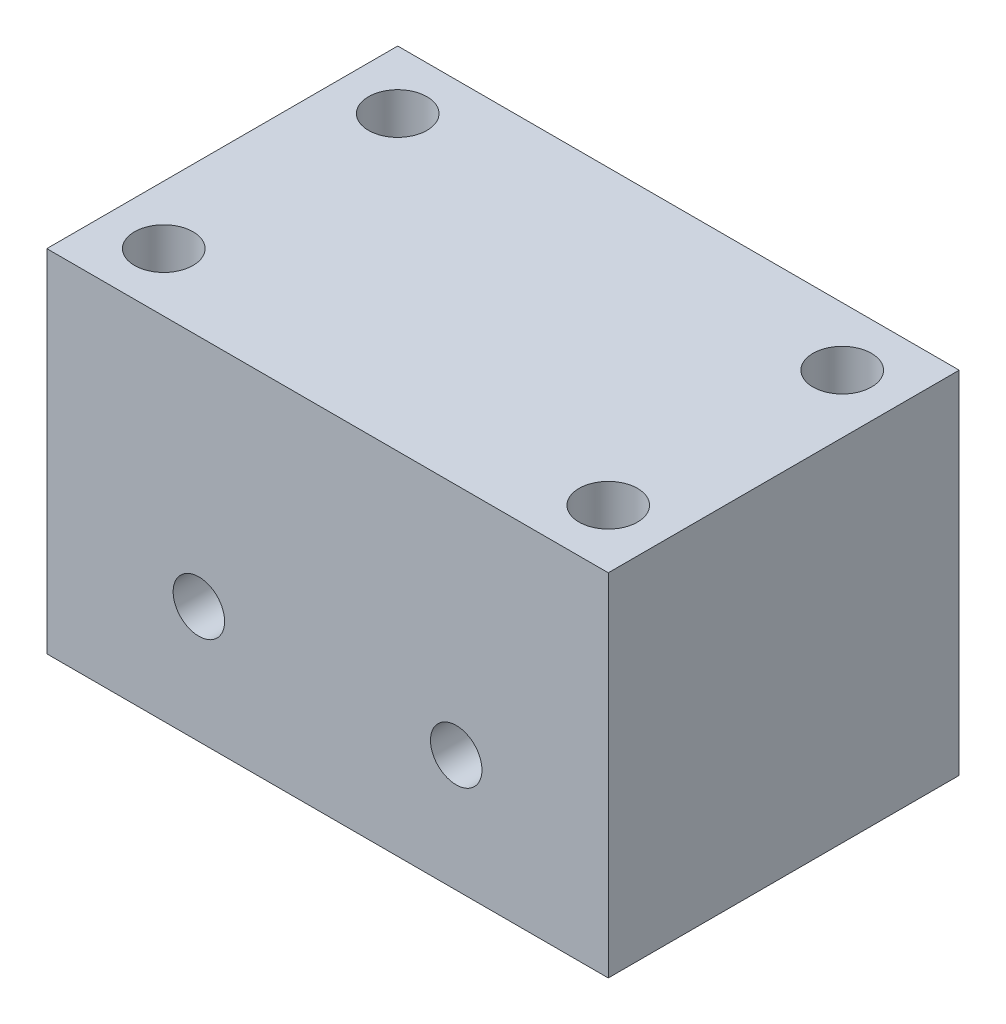
from build123d import *

# Parameters (mm, degrees)
SKETCH_1_W          = 48
SKETCH_1_H          = 30
EXTRUDE_1_DEPTH     = 30
SKETCH_2_W          = 28
SKETCH_2_H          = 15
CUT_EXTRUDE_1_DEPTH = 20
SKETCH_3_R          = 2.2
CUT_EXTRUDE_2_DEPTH = 20
SKETCH_4_R          = 2.5
CUT_EXTRUDE_3_DEPTH = 30


with BuildPart() as part:
    # 草图1 → 凸台-拉伸1 (new body)
    with BuildSketch(Plane.XY):
        with Locations((-0.545454545, 1.527272727)):
            Rectangle(SKETCH_1_W, SKETCH_1_H)
    extrude(amount=EXTRUDE_1_DEPTH)

    # 草图2 → 切除-拉伸1 (cut)
    with BuildSketch(Plane(origin=(0, 0, 0), x_dir=(-1, 0, 0), z_dir=(0, 0, -1))):
        with Locations((0.545454545, -5.972727273)):
            Rectangle(SKETCH_2_W, SKETCH_2_H)
    extrude(amount=-CUT_EXTRUDE_1_DEPTH, mode=Mode.SUBTRACT)

    # 草图3 → 切除-拉伸2 (cut)
    with BuildSketch(Plane(origin=(0, 0, 20), x_dir=(-1, 0, 0), z_dir=(0, 0, -1))):
        with Locations((-10.454545455, -3.472727273)):
            Circle(SKETCH_3_R)
        with Locations((11.545454545, -3.472727273)):
            Circle(SKETCH_3_R)
    extrude(amount=-CUT_EXTRUDE_2_DEPTH, mode=Mode.SUBTRACT)

    # 草图4 → 切除-拉伸3 (cut)
    with BuildSketch(Plane.XZ.offset(13.472727273)):
        with Locations(Location((-19.545454545, 5, 0), (0, 0, 270))):
            Circle(SKETCH_4_R)
        with Locations(Location((-19.545454545, 25, 0), (0, 0, 270))):
            Circle(SKETCH_4_R)
        with Locations(Location((18.454545455, 25, 0), (0, 0, 270))):
            Circle(SKETCH_4_R)
        with Locations(Location((18.454545455, 5, 0), (0, 0, 270))):
            Circle(SKETCH_4_R)
    extrude(amount=-CUT_EXTRUDE_3_DEPTH, mode=Mode.SUBTRACT)


solid = part.part
